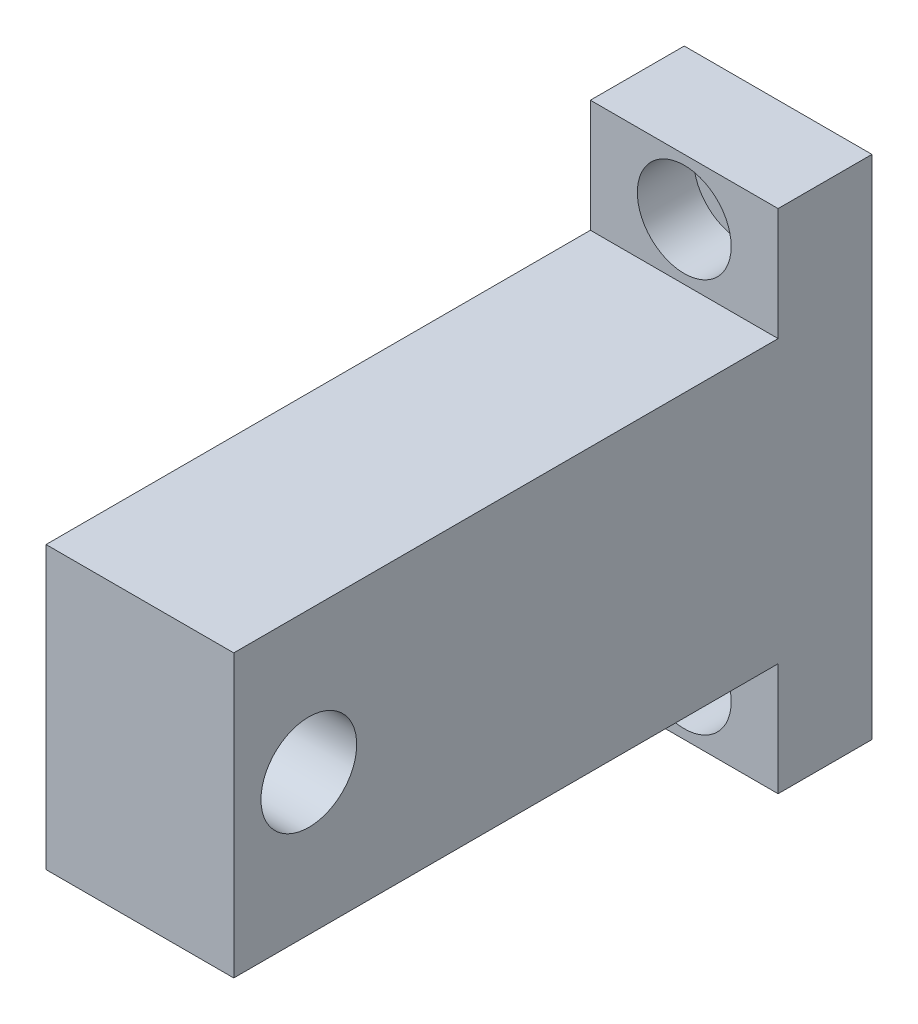
SolidWorks part; units mm, degrees
ref_plane "Front Plane" through (0, 0, 0) normal (0, 0, 1) x (1, 0, 0)
ref_plane "Top Plane" through (0, 0, 0) normal (0, 1, 0) x (1, 0, 0)
ref_plane "Right Plane" through (0, 0, 0) normal (1, 0, 0) x (0, 0, -1)
sketch "Sketch1" plane through (0, 0, 0) normal (0, 0, 1) x (1, 0, 0)
  line L0 (-36.3881, 29.6179) -> (-16.3881, 29.6179)
  line L1 (-36.3881, -24.3821) -> (-16.3881, -24.3821)
  line L2 (-16.3881, 29.6179) -> (-16.3881, -24.3821)
  line L3 (-36.3881, 29.6179) -> (-36.3881, -24.3821)
  line L4 (-36.3881, 17.6179) -> (-16.3881, 17.6179)
  line L5 (-36.3881, -12.3821) -> (-16.3881, -12.3821)
  arc A0 (-31.2781, -18.3821) -> (-21.4981, -18.3821) centre (-26.3881, -18.3821) ccw
  arc A1 (-21.4981, -18.3821) -> (-31.2781, -18.3821) centre (-26.3881, -18.3821) ccw
  arc A2 (-21.4981, 23.6179) -> (-31.2781, 23.6179) centre (-26.3881, 23.6179) ccw
  arc A3 (-31.2781, 23.6179) -> (-21.4981, 23.6179) centre (-26.3881, 23.6179) ccw
extrude "Boss-Extrude1" add sketch "Sketch1" along normal blind 10 contours L2 L1 L3 L0
sketch "Sketch2" plane through (0, 0, 10) normal (0, 0, 1) x (1, 0, 0)
  line L1 (-36.3881, 17.6179) -> (-16.3881, 17.6179)
  line L2 (-36.3881, 17.6179) -> (-36.3881, -12.3821)
  line L3 (-36.3881, -12.3821) -> (-16.3881, -12.3821)
  line L4 (-16.3881, 17.6179) -> (-16.3881, -12.3821)
extrude "Boss-Extrude2" add sketch "Sketch2" along normal blind 58
hole_wizard "CBORE for M6 Hex Head Bolt1" positions "Sketch5" profile "Sketch3" counterbore size "M6" standard "Gb" end condition through all
sketch "Sketch5" plane through (0, 0, 10) normal (0, 0, 1) x (1, 0, 0)
  point P0 (-26.3881, 23.6179)
  point P3 (-26.3881, -18.3821)
sketch "Sketch3" plane through (-26.3881, 23.6179, 10) normal (1, 0, 0) x (0, -1, 0)
  line L0 (0, 0) -> (0, 10)
  line L1 (0, 10) -> (3.3, 10)
  line L3 (3.3, 10) -> (3.3, 6)
  line L4 (3.3, 6) -> (5, 6)
  line L5 (5, 6) -> (5, 0)
  line L7 (5, 0) -> (0, 0)
  line L11 (0, -6.35) -> (0, 107.95) construction
  dimension "通孔孔直径" = 6.6
  dimension "通孔孔深度" = 10
  dimension "柱形沉头孔直径" = 10
  dimension "柱形沉头孔深度" = 6
hole_wizard "M12 Tapped Hole1" positions "Sketch7" profile "Sketch6" tap size "M12" standard "GB" end condition through all
sketch "Sketch7" plane through (-36.3881, 0, 0) normal (-1, 0, 0) x (0, 0, 1)
  line L0 (68, 2.6179) -> (20.8672, 2.6179) construction
  line L1 (68, 17.6179) -> (68, -12.3821) construction
  line L4 (0, 29.6179) -> (0, -24.3821) construction
  point P0 (60, 2.6179)
  dimension "D1" = 60
sketch "Sketch6" plane through (-36.3881, 2.6179, 60) normal (0, 1, 0) x (0, 0, 1)
  line L0 (0, 0) -> (0, 20.0001)
  line L1 (0, 20.0001) -> (5.1, 20.0001)
  line L2 (5.1, 20.0001) -> (5.1, 0)
  line L5 (5.1, 0) -> (0, 0)
  line L11 (0, -6.35) -> (0, 107.95) construction
  dimension "通孔螺纹孔钻头直径" = 10.2
  dimension "通孔螺纹孔钻头深度" = 20.0001
cosmetic thread "Cosmetic Thread1" parameters "D2"=12
